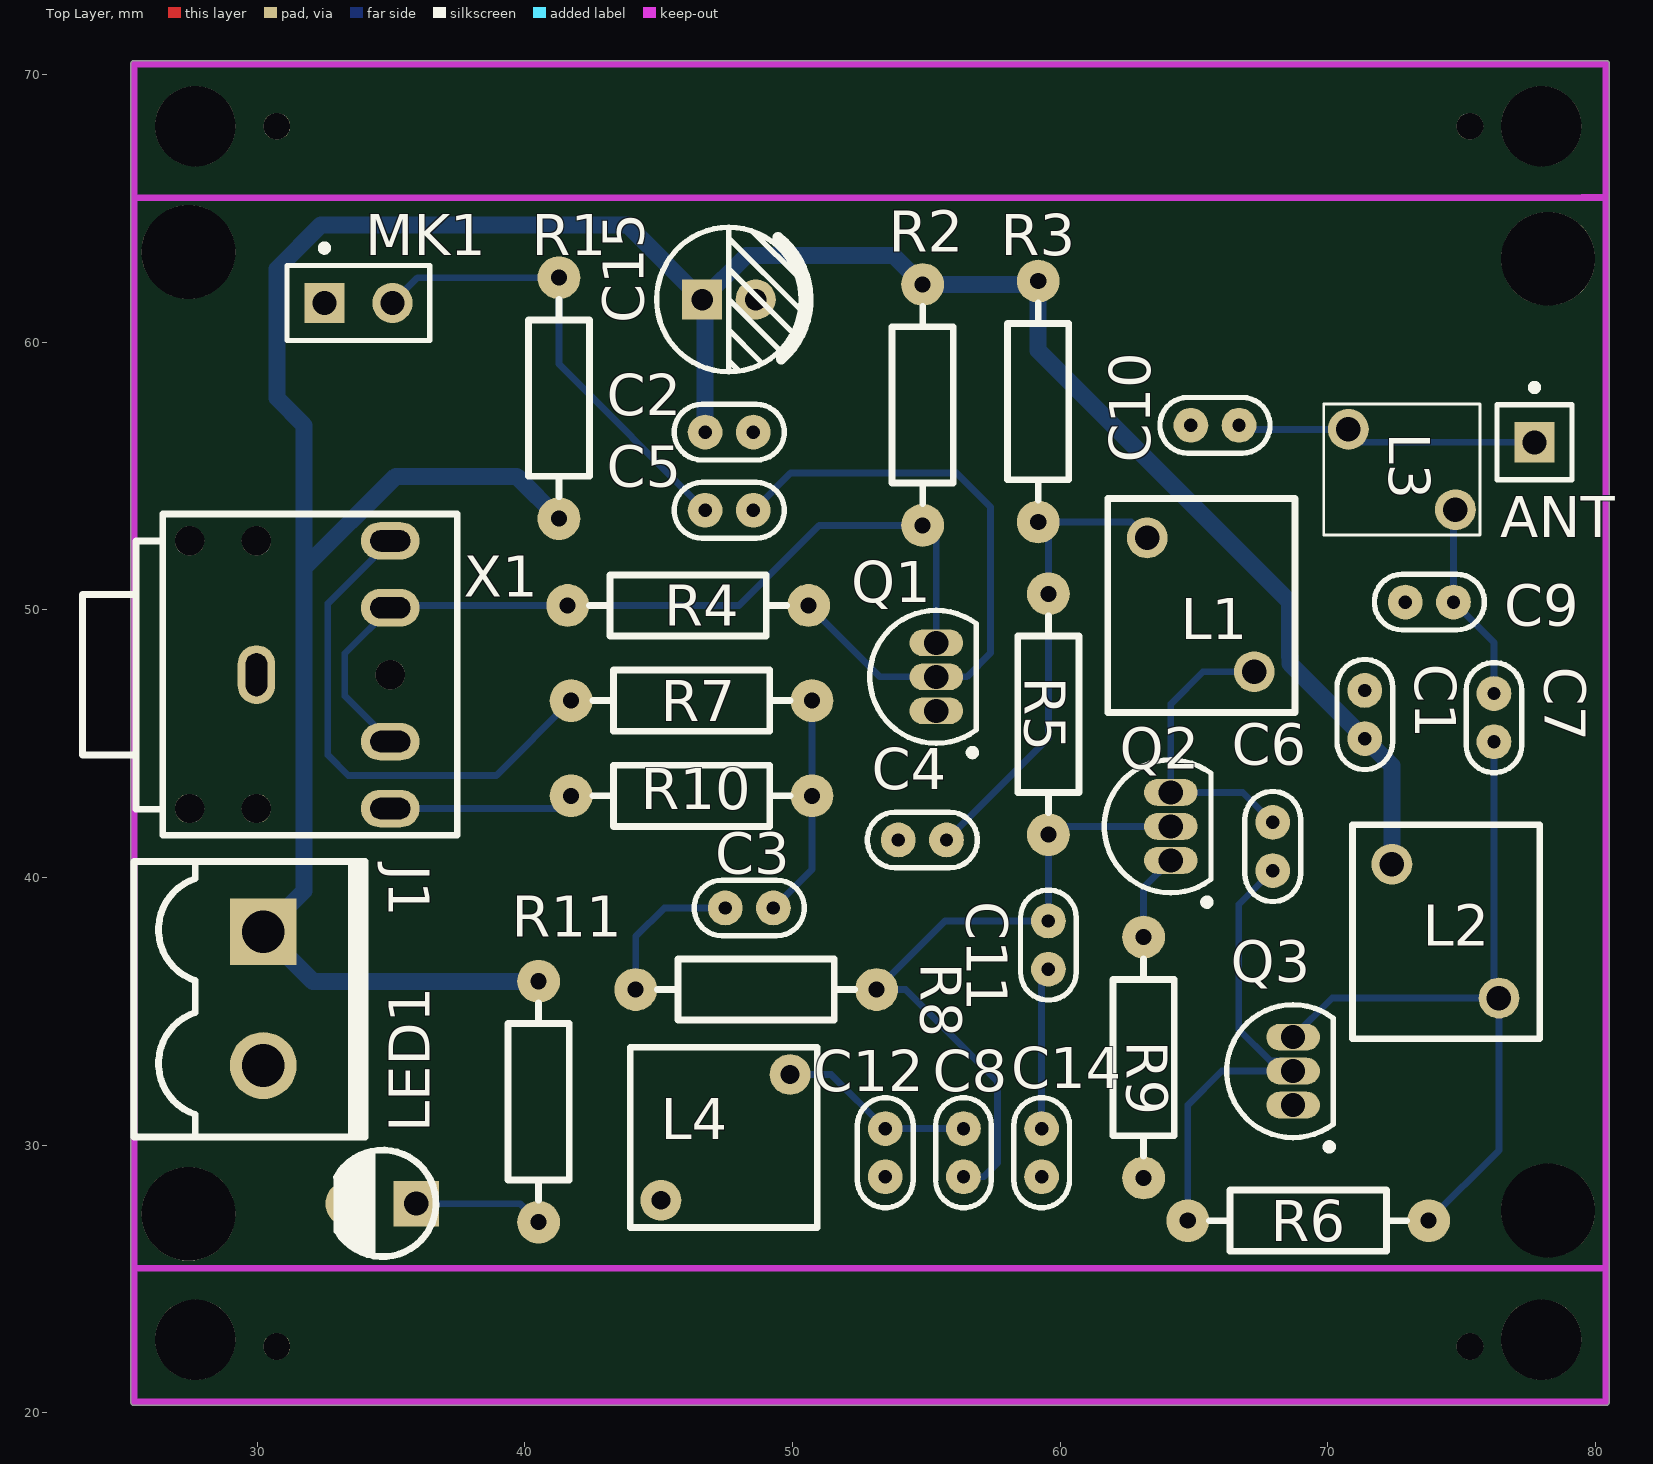
[diagram p0: Top Layer view]
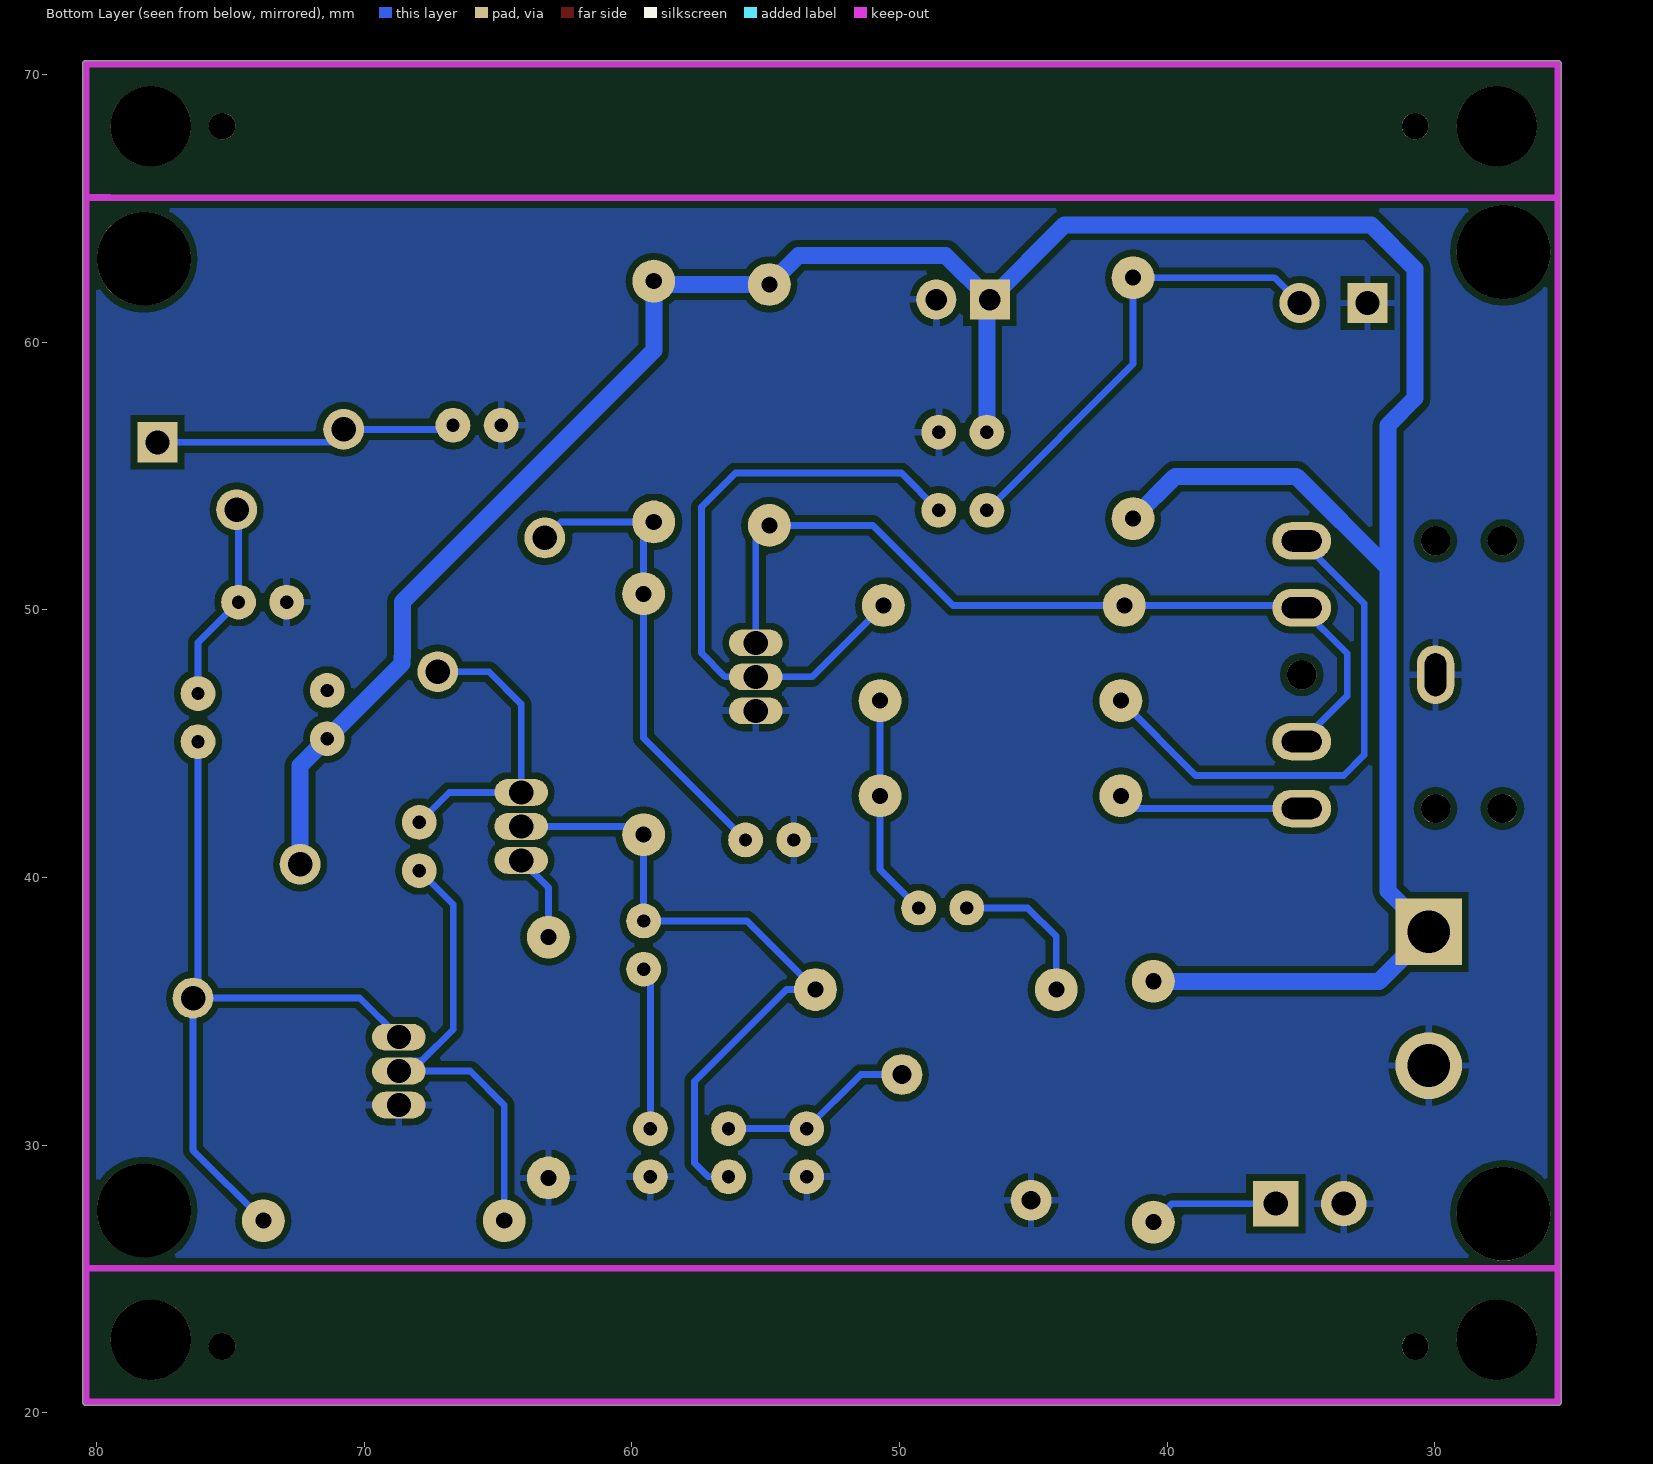
[diagram p1: Bottom Layer view, seen from below]
# Altium PCB MISC80838.PcbDoc
Units mm, origin at the board's own origin, x right, y up, seen from the top; angles counter-clockwise.
Board outline 55.25 x 50.25 mm, 2 copper layers (Top Layer, Bottom Layer); 37 components, 20 nets, 96 pads, 0 vias.

## Layer stack, top to bottom (the 12.6 mil dielectric is the usual default, probably not edited)
Top Solder: solder mask 0.0102, Solder Resist, Dk 3.5
Top Layer: signal copper 0.0356
Dielectric 1: dielectric 0.32, FR-4, Dk 4.8
Bottom Layer: signal copper 0.0356
Bottom Solder: solder mask 0.0102, Solder Resist, Dk 3.5

## Board outline
25.273,20.4 ccw(c25.4,20.4) 25.4,20.273 80.391,20.273 ccw(c80.391,20.4) 80.518,20.4 80.518,25.353 ccw(c80.4,25.4) 80.527,25.4 80.527,70.4 ccw(c80.4,70.4) 80.4,70.527 25.4,70.527 ccw(c25.4,70.4) 25.273,70.4

## Design rules (kind name [scope] priority, off if disabled: settings)
Clearance [All] p1: gap=0.254
MinimumSolderMaskSliver [All] p1: minsoldermaskwidth=0
PolygonConnect [All] p1: connectstyle=Relief reliefconductorwidth=0.254 reliefentries=4 polygonreliefangle="90 Angle" airgapwidth=0.254
RoutingVias [All] p1: holewidth=0.711 width=1.27 viastyle="Through Hole" minholewidth=0.711 minwidth=1.27 maxholewidth=0.711 maxwidth=1.27
SilkToSilkClearance [All] p1: silktosilkclearance=0
SilkToSolderMaskClearance [IsPad] p1: minsilkscreentomaskgap=0 clearancetoexposedcopper=TRUE
SolderMaskExpansion [All] p1: expansion=0.102
Width [All] p1: maxlimit=20 minlimit=0.254 preferedwidth=0.254
27 further rules are at their usual default settings.

## Components (designator, comment, footprint, x,y, rotation, side; value= is the part's Value field where it differs from the comment)
ANT "Antenna" PIN1 77.724,56.261 r0 top
C1 "102" "CC 1.8*3.6" 71.385,46.09 r270 top
C2 "104" "CC 1.8*3.6" 47.636,56.642 r180 top
C3 "104" "CC 1.8*3.6" 48.387,38.862 r180 top
C4 "102" "CC 1.8*3.6" 54.853,41.402 r0 top
C5 "104" "CC 1.8*3.6" 47.636,53.721 r0 top
C6 "101" "CC 1.8*3.6" 67.945,41.159 r90 top
C7 "30P" "CC 1.8*3.6" 76.211,45.974 r270 top
C8 "30P" "CC 1.8*3.6" 56.388,29.718 r90 top
C9 "101" "CC 1.8*3.6" 73.798,50.292 r180 top
C10 "30" "CC 1.8*3.6" 65.786,56.896 r180 top
C11 "68P" "CC 1.8*3.6" 59.563,37.476 r270 top
C12 "15P" "CC 1.8*3.6" 53.467,29.718 r270 top
C14 "101" "CC 1.8*3.6" 59.309,29.718 r270 top
C15 "47UF" "CS 2.0*5*8 - C" 47.625,61.595 r180 top
J1 "KF2EDGK-2P" KF2EDGK5.0-2P 30.226,37.973 r270 top
L1 "Air-core inductor 8T" 8T 65.278,50.165 r180 top
L2 "Air-core inductor 8T" 8T 74.422,37.973 r180 top
L3 "Air-core inductor 5T" 5T 72.771,55.245 r270 top
L4 "Adjustable inductor 7T" 可调电感7T 41.156,30.29 r0 top
LED1 "Red" "LED 3MM-B" 34.671,27.813 r180 top
MK1 "Mic2" PIN2 32.512,61.468 r0 top
Q1 "9014" TO-92A 55.372,47.498 r0 top
Q2 "9018" TO-92A 64.135,41.91 r0 top
Q3 "9018" TO-92A 68.707,32.766 r0 top
R1 "10K" "RS 1/4W" 41.275,57.912 r270 top
R2 "10K" "RS 1/4W" 54.864,57.658 r90 top
R3 "100" "RS 1/4W" 59.182,57.785 r270 top
R4 "100K" "RS 1/4W" 46.101,50.165 r0 top
R5 "47K" "RS 1/4W" 59.563,46.101 r270 top
R6 "47K" "RS 1/4W" 69.27,27.178 r180 top
R7 "10K" "RS 1/4W" 46.228,46.609 r0 top
R8 "22K" "RS 1/4W" 48.641,35.814 r0 top
R9 "470" "RS 1/4W" 63.119,33.274 r270 top
R10 "10K" "RS 1/4W" 46.228,43.053 r0 top
R11 "10K" "RS 1/4W" 40.513,31.623 r90 top
X1 "3F07" 3F07 30.472,47.578 r0 top

## Footprints (in the part's own frame and the unit in brackets; to place one, negate y for a bottom-side part, rotate by r counter-clockwise, add the part's x,y. Pads: shape width x height; smd on the part's side, far side on the other; paste and mask are expansions set on the pad)
3F07 [mm]
  oval 1.4x2.2 hole 0.8 slot 1.6 at 90 deg paste+0 mask+0.051: 1(-0.5,0)
  oval 2.2x1.4 hole 0.8 slot 1.5 at 0 deg paste+0 mask+0.051: 2(4.5,5) 3(4.5,2.5) 4(4.5,-2.5) 5(4.5,-5)
  round 1.1 hole 1.1 unplated paste+0: ""(-3,-5) ""(-3,5) ""(-0.5,-5) ""(-0.5,5) ""(4.5,0)
  silkscreen extent -7,-6 7,6
5T [mil]
  round 60 hole 36 paste+4 mask+4: 1(-59.05,-78.74) 2(59.05,78.74)
  silkscreen extent -96,-115 96,115
8T [mil]
  round 60 hole 36 paste+0 mask+2: 1(-77.8,97.48) 2(79.68,-99.37)
  silkscreen extent -138,-157 138,157
"CC 1.8*3.6" [mm] "脚距1.8mm直径3.6mm"
  round 1.3 hole 0.5: 1(-0.9,0) 2(0.9,0)
  silkscreen extent -2.05,-1.04 2.05,1.04, body extent -1.8,-0.8 1.8,0.8, height 3.6
"CS 2.0*5*8 - C" [mm] "脚距2mm , 直径5mm , 高8mm"
  rect 1.5x1.5 hole 0.8: 1(1,0)
  round 1.5 hole 0.8: 2(-1,0)
  silkscreen extent -2.96,-2.7 2.7,2.7, body extent -2.5,-2.5 2.5,2.5, height 8.02
KF2EDGK5.0-2P [mm]
  rect 2.5x2.5 hole 1.6: 1(0,0)
  round 2.5 hole 1.6: 2(5,0)
  silkscreen extent -2.62,-4.83 7.67,3.81, body extent -2.54,-4.76 7.54,3.74, height 11.25
"LED 3MM-B" [mm] "蓝色3mm直插LED"
  rect 1.7x1.7 hole 0.9: 1(-1.27,0)
  round 1.7 hole 0.9: 2(1.27,0)
  silkscreen extent -2.01,-2 1.72,1.98, body extent -1.95,-1.95 1.64,1.95, height 5.55
PIN1 [mm] "Generic Antenna; 1 Lead"
  rect 1.5x1.5 hole 0.9: 1(0,0)
  silkscreen extent -1.4,-1.4 1.4,2.17
PIN2 [mm] "Photosensitive Diode; 2 Leads"
  rect 1.5x1.5 hole 0.9: 1(0,0)
  round 1.5 hole 0.9: 2(2.54,0)
  silkscreen extent -1.4,-1.4 3.94,2.17
"RS 1/4W" [mm] "直插色环电阻，脚距9mm，直径2.3mm"
  round 1.6 hole 0.6: 1(-4.5,0) 2(4.5,0)
  silkscreen extent -3.68,-1.14 3.68,1.14, body extent -4.72,-1.16 4.73,1.16, height 2.32
TO-92A [mm] "TO, Flat Index; 3 In-Line, Axial Leads; Body Dia. 4.5mm; Leads 0.51 x 0.48 mm (max)"
  oval 2x1 hole 0.9: 1(0,-1.27) 2(0,0) 3(0,1.27)
  silkscreen extent -2.48,-2.95 1.5,2.48, body extent -2.48,-2.5 1.5,2.5, height 6.86
可调电感7T [mil]
  round 60 hole 27.56 paste+0 mask+2: 1(154.68,-92.5) 2(344.68,92.49)
  silkscreen extent 110,-132 385,132

## Part data
ANT: "Generic Antenna"
C1 C2 C3 C4 C5 C6 C7 C8 C9 C10 C11 C12 C14: library part CC, "Ceramic capacitor"
C15: library part CS, "Through-hole solid-state capacitor"
L1 L2: library part INDUCTOR
L3: library part 空心电感5T, "INDUCTOR"
L4: library part IND_ADJ
LED1: library part LED-3MM, "Through-hole 3mm LED"
MK1: "Microphone"
Q1 Q2 Q3: library part 2N3904, "NPN General Purpose Amplifier"
R1 R2 R3 R4 R5 R6 R7 R8 R9 R10 R11: library part R-S, "Color-band resistor"

## Free pads (board coordinates)
  round 3.5 hole 3.5: 0(27.432,63.373) 1(27.432,27.432) 2(78.232,27.559) 3(78.232,63.119)
  round 3 hole 3: 4(27.686,22.733) 4(27.686,68.072) 4(77.978,22.733) 5(77.978,68.072)
  round 1 hole 1: 6(30.734,68.072) 7(75.311,68.072) 8(75.311,22.479) 9(30.734,22.479)

## Nets (pads, with @x,y where several pads share a name; then routed paths per layer and width w, separated by ;. In a path a pad name is that pad's centre, name@x,y a point inside that pad or via, vN(x,y) a via of type N, cw(c..) or ccw(c..) an arc to the next point about the centre after c; other vN are vias at no path point)
GND: C2.1 C4.1 C9.2 C10.2 C12.2 C14.2 C15.2 J1.2 L4.1 LED1.2 MK1.1 Q1.1 Q3.1 R9.2 X1.1
NetANT_1: ANT.1 C10.1 L3.1 | length 11.3
  Bottom Layer w0.254: C10.1 66.837,56.745 L3.1 71.255,56.261 ANT.1
NetC3_1: C3.1 R7.2 R10.2 | length 8.3
  Bottom Layer w0.254: C3.1 50.728,40.303 R10.2 R7.2
NetC3_2: C3.2 R8.1 | length 5.8
  Bottom Layer w0.254: R8.1 44.141,37.791 45.212,38.862 C3.2
NetC4_2: C4.2 L1.2 R3.2 R5.1 | length 17.9
  Bottom Layer w0.254: C4.2 59.563,45.212 R5.1 59.563,52.904 R3.2 62.658,53.285 L1.2
NetC5_1: C5.1 MK1.2 R1.1 | length 17.6
  Bottom Layer w0.254: MK1.2 35.996,62.412 R1.1 41.275,59.182 C5.1
NetC5_2: C5.2 Q1.2 R4.2 | length 23.7
  Bottom Layer w0.254: C5.2 49.933,55.118 56.134,55.118 57.404,53.848 57.404,48.387 56.515,47.498 Q1.2 53.268,47.498 R4.2
NetC6_1: C6.1 Q3.2 R6.2 | length 17.9
  Bottom Layer w0.254: R6.2 64.77,31.496 66.04,32.766 Q3.2 68.318,33.155 67.842,33.155 66.675,34.322 66.675,38.989 C6.1
NetC6_2: C6.2 L1.1 Q2.3 | length 11.2
  Bottom Layer w0.254: L1.1 65.342,47.689 64.135,46.482 Q2.3 66.824,43.18 C6.2
NetC7_1: C7.1 C9.1 L3.2 | length 7.5
  Bottom Layer w0.254: L3.2 74.698,53.672 C9.1 76.211,48.779 C7.1
NetC7_2: C7.2 L2.1 Q3.3 R6.1 | length 27.4
  Bottom Layer w0.254: Q3.3 70.168,35.497 L2.1 ; R6.1 76.398,29.806 L2.1 ; C7.2 76.211,35.684 L2.1
NetC8_1: C8.1 C11.1 Q2.2 R5.2 R8.2 | length 25.9
  Bottom Layer w0.254: C8.1 57.139,28.818 57.658,29.337 57.658,32.385 54.229,35.814 R8.2 55.703,38.376 C11.1 R5.2 59.872,41.91 Q2.2
NetC8_2: C8.2 C12.1 L4.2 | length 7.3
  Bottom Layer w0.254: L4.2 51.446,32.639 C12.1 C8.2
NetC11_2: C11.2 C14.1 | length 6.1
  Bottom Layer w0.254: C14.1 59.309,36.322 C11.2
NetLED1_1: LED1.1 R11.1 | length 4.9
  Bottom Layer w0.254: LED1.1 39.823,27.813 R11.1
NetQ1_3: Q1.3 R2.1 R4.1 X1.3 X1.4 | length 32.2
  Bottom Layer w0.254: X1.4 33.274,46.776 33.274,48.38 X1.3 35.059,50.165 R4.1 48.006,50.165 50.999,53.158 R2.1 55.372,52.65 Q1.3
NetQ2_1: Q2.1 R9.1 | length 3.3
  Bottom Layer w0.254: R9.1 63.119,39.624 Q2.1
NetR7_1: R7.1 X1.2 | length 19.5
  Bottom Layer w0.254: X1.2 32.639,50.245 32.639,44.577 33.401,43.815 38.934,43.815 R7.1
NetR10_1: R10.1 X1.5 | length 7
  Bottom Layer w0.254: X1.5 41.253,42.578 R10.1
VCC: C1.2 C2.2 C15.1 J1.1 L2.2 R1.2 R2.2 R3.1 R11.2 | length 112.2
  Bottom Layer w0.635: R11.2 32.076,36.123 J1.1 31.75,39.497 31.75,51.562 ; R1.2 39.696,54.991 35.179,54.991 31.75,51.562 ; C2.2 46.736,61.484 C15.1 ; L2.2 72.398,44.177 C1.2 68.587,47.988 68.587,48.249 68.58,48.256 68.58,50.292 59.182,59.69 R3.1 59.055,62.158 R2.2 53.776,63.246 48.276,63.246 C15.1 ; 31.75,51.562 31.75,56.896 30.734,57.912 30.734,62.738 32.385,64.389 43.831,64.389 C15.1
pads on no net: C1.1 X1.

## Polygon pours and split planes (outlines as drawn)
GND on Bottom Layer "G" (solid, remove dead copper, pour order 0): 17.399,69.977 17.78,70.358 86.487,70.358 86.487,22.352 85.725,21.59 84.582,22.733 16.129,22.733

## Keep-outs
Keep-Out Layer:
  lines w0.254: 79.502,65.4 cw(c79.514,65.388) 79.514,65.405 80.4,65.405 ; 79.883,65.405 cw(c79.871,65.417) 79.871,65.4 25.4,65.4 ; 80.391,25.4 80.391,20.4 25.4,20.4 25.4,25.4 ; 80.391,65.405 cw(c80.369,65.383) 80.4,65.383 ; 80.391,67.056 cw(c80.369,67.034) 80.4,67.034 ; 25.4,25.4 80.4,25.4 80.4,65.405 ; 25.4,25.4 25.4,65.4 ; 25.4,65.4 25.4,70.4 80.4,70.4 80.4,65.405